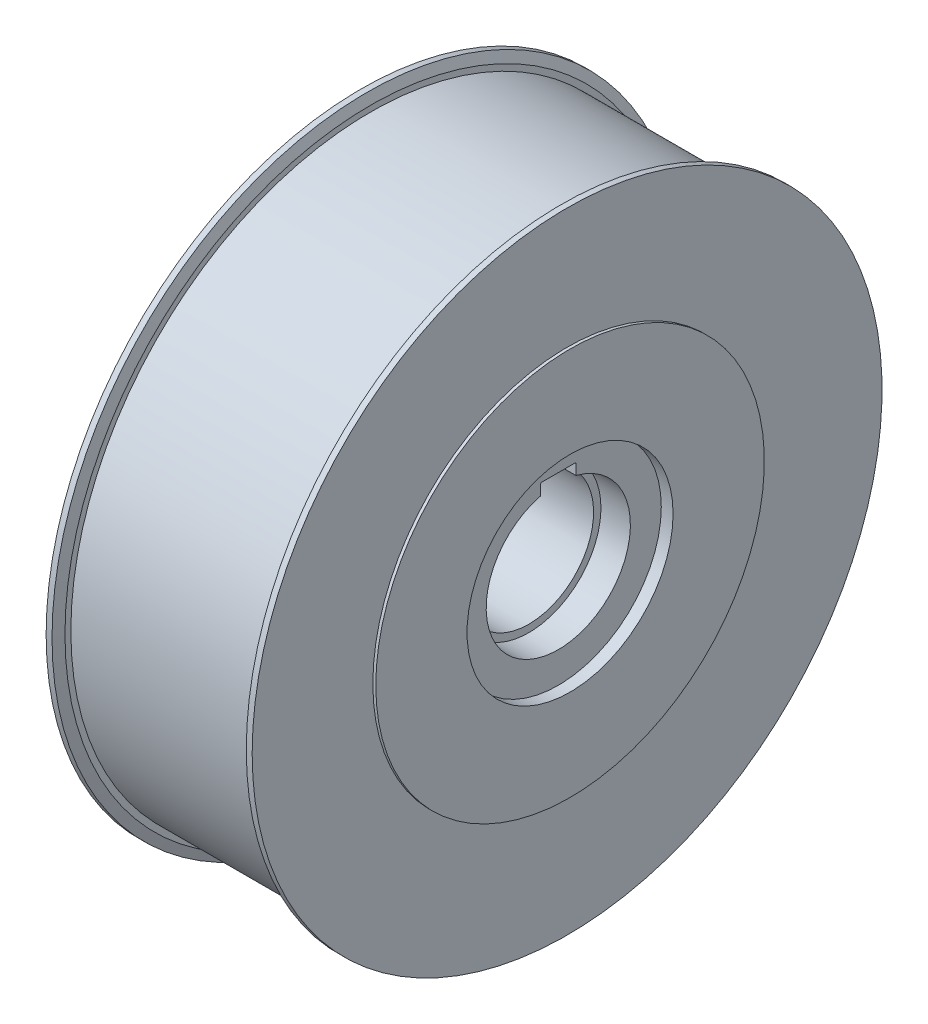
SolidWorks part; units mm, degrees
ref_plane "Front Plane" through (0, 0, 0) normal (0, 0, 1) x (1, 0, 0)
ref_plane "Top Plane" through (0, 0, 0) normal (0, 1, 0) x (1, 0, 0)
ref_plane "Right Plane" through (0, 0, 0) normal (1, 0, 0) x (0, 0, -1)
sketch "Sketch1" plane through (0, 0, 0) normal (0, 0, 1) x (1, 0, 0)
  line L0 (0, 0) -> (24.34, 0) construction
  line L1 (-18, 0) -> (-18, 33)
  line L2 (-18, 33) -> (-17.5, 33)
  line L3 (-17.5, 33) -> (-17.5, 53.5)
  line L4 (-17.5, 53.5) -> (-16.5, 53.5)
  line L5 (-16.5, 53.5) -> (-15.9, 51.9)
  line L6 (-15.9, 50.9) -> (15.9, 50.9)
  line L7 (-15.9, 51.9) -> (-15.9, 50.9)
  line L8 (18, 0) -> (18, 33)
  line L9 (0, -14.9938) -> (0, 64.0343) construction
  line L10 (18, 33) -> (17.5, 33)
  line L11 (17.5, 33) -> (17.5, 53.5)
  line L12 (17.5, 53.5) -> (16.5, 53.5)
  line L13 (16.5, 53.5) -> (15.9, 51.9)
  line L14 (15.9, 51.9) -> (15.9, 50.9)
  line L16 (-18, 0) -> (18, 0)
  point P21 (0, 50.9)
  dimension "D1" = 53.5
  dimension "D2" = 33
  dimension "D3" = 18
  dimension "D4" = 0.5
  dimension "D5" = 2.6
  dimension "D6" = 1
  dimension "D7" = 1
  dimension "D8" = 1.6
revolve "Revolve1" add sketch "Sketch1" angle 360 about L16
sketch "Sketch2" plane through (18, 0, 0) normal (1, 0, 0) x (0, 0, -1)
  circle A0 centre (0, 0) radius 17.5
extrude "Cut-Extrude1" cut sketch "Sketch2" against normal blind 2
sketch "Sketch3" plane through (16, 0, 0) normal (1, 0, 0) x (0, 0, -1)
  line L0 (3, 10.583) -> (3, 13.8)
  line L2 (-3, 10.583) -> (-3, 13.8)
  line L3 (-3, 13.8) -> (3, 13.8)
  arc A0 (-3, 10.583) -> (3, 10.583) centre (0, 0) ccw
  dimension "D1" = 6
  dimension "D3" = 22
  dimension "D2" = 13.8
extrude "Cut-Extrude2" cut sketch "Sketch3" against normal through all
sketch "Sketch4" plane through (16, 0, 0) normal (1, 0, 0) x (0, 0, -1)
  circle A0 centre (0, 0) radius 12.25
extrude "Cut-Extrude3" cut sketch "Sketch4" against normal blind 5
fillet "Fillet1" radius 0.2 2 edges at (-1, 13.8, -3) (-1, 13.8, 3)
